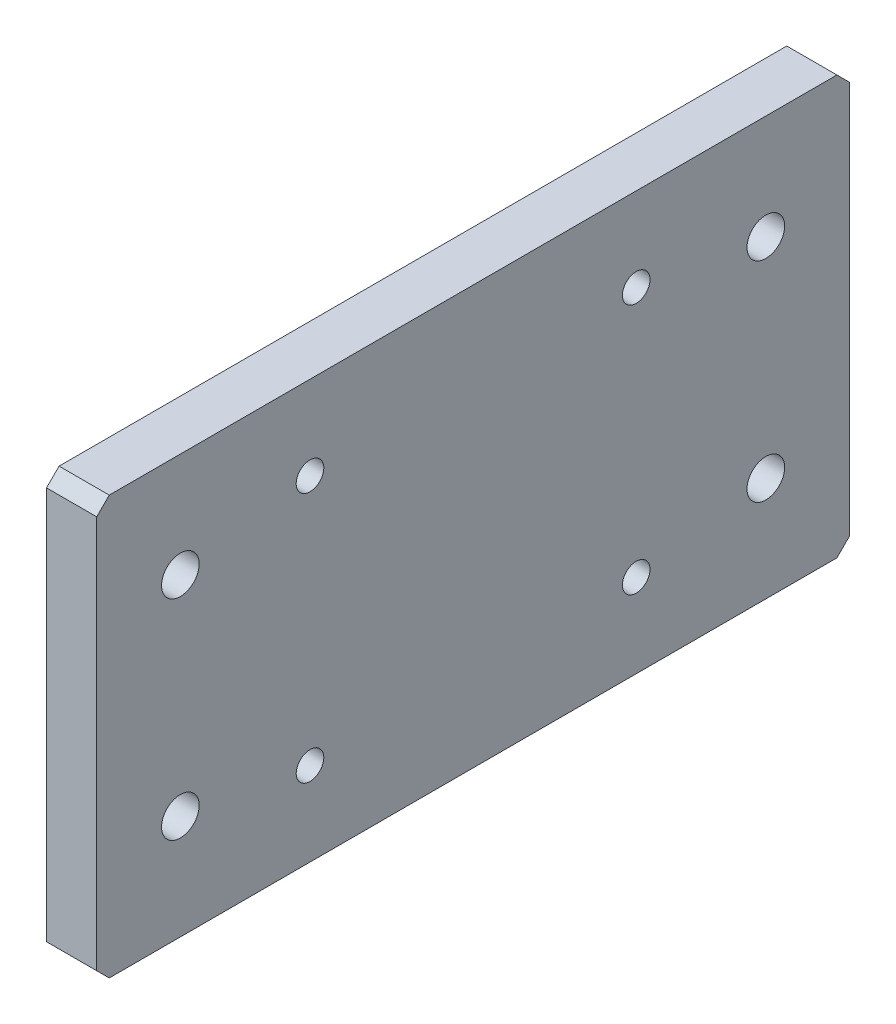
SolidWorks part; units mm, degrees
ref_plane "前视基准面" through (0, 0, 0) normal (0, 0, 1) x (1, 0, 0)
ref_plane "上视基准面" through (0, 0, 0) normal (0, 1, 0) x (1, 0, 0)
ref_plane "右视基准面" through (0, 0, 0) normal (1, 0, 0) x (0, 0, -1)
sketch "草图1" plane through (0, 0, 0) normal (1, 0, 0) x (0, 0, -1)
  line L1 (-90, 50) -> (90, 50)
  line L2 (-90, 50) -> (-90, -50)
  line L3 (-90, -50) -> (90, -50)
  line L4 (90, 50) -> (90, -50)
  line L5 (-90, 50) -> (90, -50) construction
  line L6 (-90, -50) -> (90, 50) construction
  point P0 (0, 0)
  dimension "D1" = 180
  dimension "D2" = 100
extrude "凸台-拉伸1" add sketch "草图1" along normal blind 12
hole_wizard "打孔尺寸(%根据)内六角圆柱头螺钉的类型1" positions "草图2" profile "草图3" counterbore size "M6" standard "GB" end condition through all
sketch "草图2" plane through (0, 0, 0) normal (-1, 0, 0) x (0, 0, 1)
  line L0 (0, 113.6431) -> (0, 0) construction
  line L1 (0, 0) -> (148.5259, 0) construction
  point P0 (-39, 30)
  point P2 (-39, -30)
  point P4 (39, 30)
  point P6 (39, -30)
  dimension "D1" = 60
  dimension "D2" = 78
sketch "草图3" plane through (0, 30, -39) normal (0, 1, 0) x (0, 0, 1)
  line L0 (0, 0) -> (0, 12)
  line L1 (0, 12) -> (3.3, 12)
  line L3 (3.3, 12) -> (3.3, 6.8)
  line L4 (3.3, 6.8) -> (5.5, 6.8)
  line L5 (5.5, 6.8) -> (5.5, 0)
  line L7 (5.5, 0) -> (0, 0)
  line L11 (0, -6.35) -> (0, 107.95) construction
  dimension "通孔孔直径" = 6.6
  dimension "通孔孔深度" = 12
  dimension "柱形沉头孔直径" = 11
  dimension "柱形沉头孔深度" = 6.8
hole_wizard "Ø9.0 (9) 直径孔1" positions "草图4" profile "草图5" hole size "Ø9.0" standard "GB" end condition through all
sketch "草图4" plane through (0, 0, 0) normal (-1, 0, 0) x (0, 0, 1)
  line L0 (0, 97.5255) -> (0, 0) construction
  line L1 (0, 0) -> (135.5254, 0) construction
  point P0 (-70, 25)
  point P2 (-70, -25)
  point P4 (70, 25)
  point P6 (70, -25)
  dimension "D1" = 50
  dimension "D2" = 140
sketch "草图5" plane through (0, 25, -70) normal (0, 1, 0) x (0, 0, 1)
  line L0 (0, 0) -> (0, 12)
  line L1 (0, 12) -> (4.5, 12)
  line L2 (4.5, 12) -> (4.5, 0)
  line L5 (4.5, 0) -> (0, 0)
  line L11 (0, -6.35) -> (0, 107.95) construction
  dimension "通孔孔直径" = 9
  dimension "通孔孔深度" = 12
chamfer "倒角1" distance 3 angle 45 4 edges at (6, 50, 90) (6, -50, 90) (6, 50, -90) (6, -50, -90)
